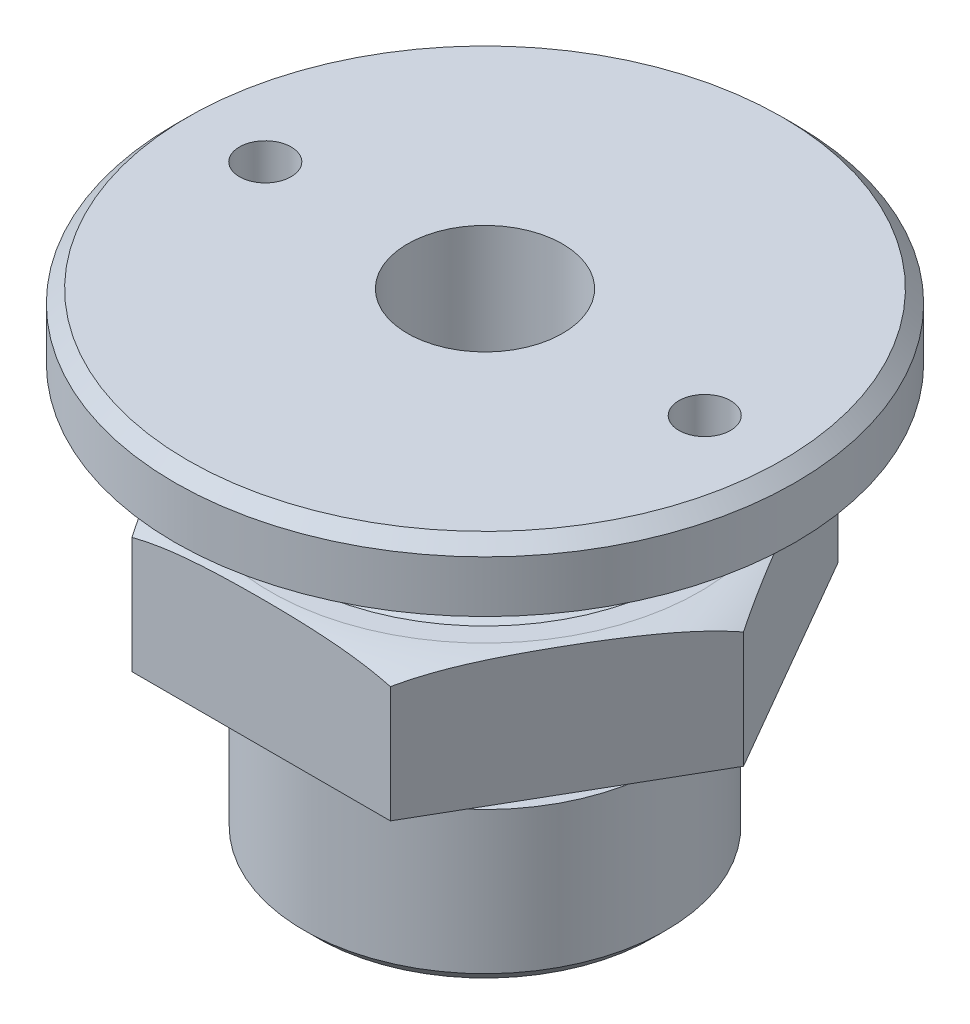
SolidWorks part; units mm, degrees
ref_plane "Front" through (0, 0, 0) normal (0, 0, 1) x (1, 0, 0)
ref_plane "Top" through (0, 0, 0) normal (0, 1, 0) x (1, 0, 0)
ref_plane "Right" through (0, 0, 0) normal (1, 0, 0) x (0, 0, -1)
sketch "Sketch1" plane through (0, 0, 0) normal (0, 0, 1) x (1, 0, 0)
  line L0 (6, 0) -> (6, 37)
  line L1 (6, 37) -> (24, 37)
  line L2 (24, 37) -> (24, 32)
  line L3 (24, 32) -> (14, 32)
  line L4 (6, 0) -> (14, 0)
  line L5 (14, 0) -> (14, 12)
  line L6 (14, 12) -> (10, 12)
  line L7 (10, 12) -> (10, 15)
  line L8 (10, 15) -> (20, 15)
  line L9 (20, 15) -> (20, 25)
  line L10 (20, 25) -> (15, 25)
  line L11 (0, 0) -> (0, 45.5015) construction
  arc A0 (14, 32) -> (15, 25) centre (16.352, 28.7646) ccw
  dimension "D13" = 4
  dimension "D1" = 6
  dimension "D2" = 37
  dimension "D3" = 18
  dimension "D4" = 5
  dimension "D5" = 10
  dimension "D6" = 8
  dimension "D7" = 12
  dimension "D8" = 4
  dimension "D9" = 3
  dimension "D10" = 10
  dimension "D11" = 10
  dimension "D12" = 5
revolve "Revolve2" add sketch "Sketch1" angle 360 about L11
chamfer "Chamfer2" distance 1 angle 45 1 edges at (0, 0, -14)
sketch "Sketch2" plane through (0, 25, 0) normal (0, 1, 0) x (1, 0, 0)
  line L1 (20, 0) -> (10, 17.3205)
  line L2 (10, 17.3205) -> (-10, 17.3205)
  line L3 (-10, 17.3205) -> (-20, 0)
  line L4 (-20, 0) -> (-10, -17.3205)
  line L5 (-10, -17.3205) -> (10, -17.3205)
  line L6 (10, -17.3205) -> (20, 0)
  circle A0 centre (0, 0) radius 17.3205 construction
  circle A1 centre (0, 0) radius 31.3788
  dimension "D1" = 40
extrude "Cut-Extrude1" cut sketch "Sketch2" against normal up to next
sketch "Sketch3" plane through (0, 0, 0) normal (0, 0, 1) x (1, 0, 0)
  line L0 (0, 0) -> (0, 42.654) construction
  line L1 (-20, 15) -> (-20, 25) construction
  line L3 (-20, 24) -> (-20, 25)
  line L5 (-20, 25) -> (-16.6145, 25)
  arc A0 (-20, 24) -> (-16.6145, 25) centre (-15.8073, 16.0363) cw
  dimension "D3" = 1
  dimension "D1" = 9
revolve "Cut-Revolve1" cut sketch "Sketch3" angle 360 about L0
chamfer "Chamfer3" distance 1 angle 45 1 edges at (0, 37, -24)
sketch "Sketch4" plane through (0, 37, 0) normal (0, 1, 0) x (1, 0, 0)
  line L0 (0, 0) -> (0, 16.9283) construction
  line L1 (0, 0) -> (29.1445, 0) construction
  circle A0 centre (17, 0) radius 2
  circle A1 centre (-17, 0) radius 2
extrude "Cut-Extrude2" cut sketch "Sketch4" against normal up to next
scale "Scale 1" bodies to scale 105 scale about centroid uniform scaling yes scale factor 1.875
